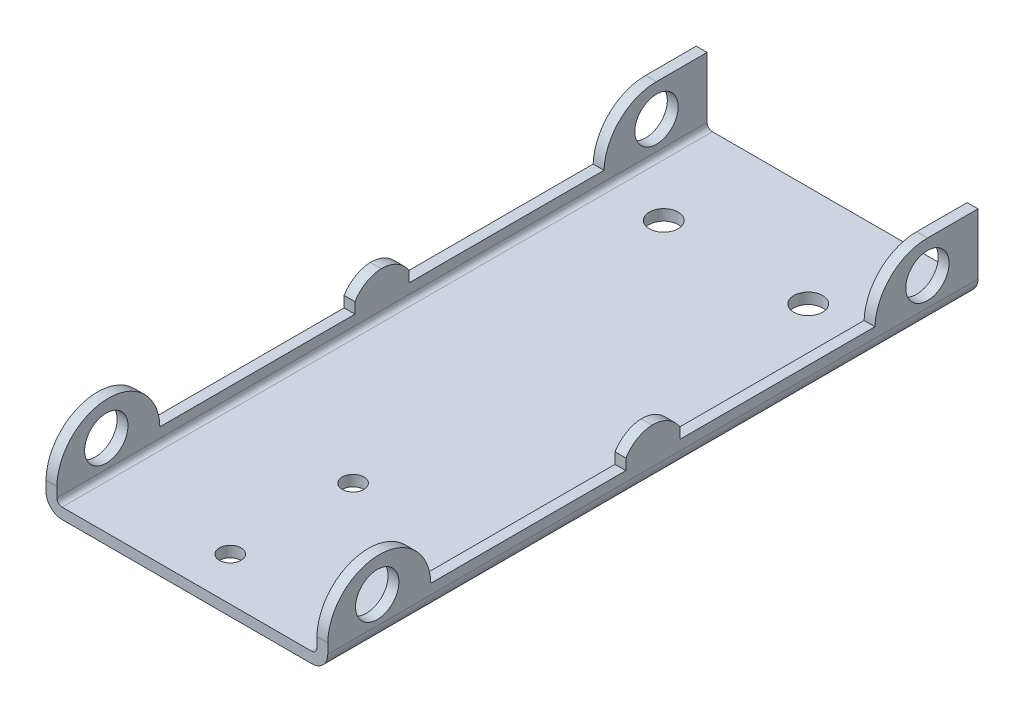
SolidWorks part; units mm, degrees
ref_plane "Front Plane" through (0, 0, 0) normal (0, 0, 1) x (1, 0, 0)
ref_plane "Top Plane" through (0, 0, 0) normal (0, 1, 0) x (1, 0, 0)
ref_plane "Right Plane" through (0, 0, 0) normal (1, 0, 0) x (0, 0, -1)
other "Configuration Table"
ref_plane "Plane1" through (-29, 0, 0) normal (-1, 0, 0) x (0, -1, 0)
sketch "Sketch1" plane through (-29, 0, 0) normal (-1, 0, 0) x (0, -1, 0)
  line L0 (-9.1381, -90) -> (1.5, -90)
  line L1 (1.5, -90) -> (1.5, 0)
  line L2 (1.5, 0) -> (-2.1289, 0)
  line L3 (-2.1289, -14.2617) -> (-2.1289, -41.2617)
  line L4 (-2.1289, -41.2617) -> (-3.6289, -41.2617)
  line L5 (-3.6383, -48.7314) -> (-2.1381, -48.7314)
  line L6 (-2.1381, -48.7314) -> (-2.1381, -75.7314)
  line L7 (-9.1381, -83) -> (-9.1381, -90)
  arc A0 (-2.1289, 0) -> (-2.1289, -14.2617) centre (-1.998, -7.1309) ccw
  arc A1 (-3.6289, -41.2617) -> (-5.7783, -44.8732) centre (-1.2572, -45.1185) ccw
  arc A2 (-5.7783, -44.8732) -> (-3.6383, -48.7314) centre (-1.2506, -44.8845) ccw
  arc A3 (-2.1381, -75.7314) -> (-9.1381, -83) centre (-1.8643, -83) ccw
extrude "Boss-Extrude1" add sketch "Sketch1" against normal blind 1.5
sketch "Sketch2" plane through (-27.5, 0, 0) normal (1, 0, 0) x (0, 0, -1)
  line L0 (0, 0) -> (90, 0)
  line L1 (90, 0) -> (90, -1.5)
  line L2 (90, -1.5) -> (0, -1.5)
  line L3 (0, -1.5) -> (0, 0)
extrude "Boss-Extrude2" add sketch "Sketch2" along normal blind 36
sketch "Sketch3" plane through (8.5, 0, 0) normal (1, 0, 0) x (0, 0, -1)
  line L0 (0, -1.5) -> (0, 2.1289)
  line L1 (14.2617, 2.1289) -> (41.2617, 2.1289)
  line L2 (41.2617, 2.1289) -> (41.2617, 3.6289)
  line L3 (48.7314, 3.6383) -> (48.7314, 2.1381)
  line L4 (48.7314, 2.1381) -> (75.7314, 2.1381)
  line L5 (83, 9.1381) -> (90, 9.1381)
  line L6 (90, 9.1381) -> (90, -1.5)
  line L7 (90, -1.5) -> (0, -1.5)
  arc A0 (0, 2.1289) -> (14.2617, 2.1289) centre (7.1309, 1.998) cw
  arc A1 (41.2617, 3.6289) -> (44.8732, 5.7783) centre (45.1185, 1.2572) cw
  arc A2 (44.8732, 5.7783) -> (48.7314, 3.6383) centre (44.8845, 1.2506) cw
  arc A3 (75.7314, 2.1381) -> (83, 9.1381) centre (83, 1.8643) cw
extrude "Boss-Extrude3" add sketch "Sketch3" along normal blind 1.5
hole_wizard "Ø6.0 (6) Diameter Hole1" positions "Sketch5" profile "Sketch4" hole size "Ø6.0" standard "ANSI Metric"
sketch "Sketch5" plane through (8.5, 0, 0) normal (-1, 0, 0) x (0, 0, 1)
  point P0 (-6.8458, 4.4817)
  point P1 (-83, 4.6381)
sketch "Sketch4" plane through (8.5, 4.4817, -6.8458) normal (0, 1, 0) x (0, 0, 1)
  line L0 (0, 0) -> (0, 1.5)
  line L1 (0, 1.5) -> (3, 1.5)
  line L2 (3, 1.5) -> (3, 0)
  line L5 (3, 0) -> (0, 0)
  line L11 (0, -6.35) -> (0, 107.95) construction
  dimension "通孔孔直径" = 6
  dimension "通孔孔深度" = 1.5
hole_wizard "Ø6.0 (6) Diameter Hole2" positions "Sketch7" profile "Sketch6" hole size "Ø6.0" standard "ANSI Metric"
sketch "Sketch7" plane through (-27.5, 0, 0) normal (1, 0, 0) x (0, 0, -1)
  point P0 (83, 4.6381)
  point P1 (6.8458, 4.4817)
sketch "Sketch6" plane through (-27.5, 4.6381, -83) normal (0, 1, 0) x (0, 0, -1)
  line L0 (0, 0) -> (0, 1.5)
  line L1 (0, 1.5) -> (3, 1.5)
  line L2 (3, 1.5) -> (3, 0)
  line L5 (3, 0) -> (0, 0)
  line L11 (0, -6.35) -> (0, 107.95) construction
  dimension "通孔孔直径" = 6
  dimension "通孔孔深度" = 1.5
hole_wizard "Ø4.0 (4) Diameter Hole1" positions "Sketch9" profile "Sketch8" hole size "Ø4.0" standard "ANSI Metric"
sketch "Sketch9" plane through (0, 0, 0) normal (0, 1, 0) x (1, 0, 0)
  point P0 (-19.5, 76)
  point P1 (0.5, 76)
sketch "Sketch8" plane through (-19.5, 0, -76) normal (1, 0, 0) x (0, 0, 1)
  line L0 (0, 0) -> (0, 1.5)
  line L1 (0, 1.5) -> (2, 1.5)
  line L2 (2, 1.5) -> (2, 0)
  line L5 (2, 0) -> (0, 0)
  line L11 (0, -6.35) -> (0, 107.95) construction
  dimension "通孔孔直径" = 4
  dimension "通孔孔深度" = 1.5
hole_wizard "Ø3.0 (3) Diameter Hole1" positions "Sketch11" profile "Sketch10" hole size "Ø3.0" standard "ANSI Metric"
sketch "Sketch11" plane through (0, 0, 0) normal (0, 1, 0) x (1, 0, 0)
  point P0 (-9.5, 6)
  point P1 (-9.5, 23)
sketch "Sketch10" plane through (-9.5, 0, -6) normal (1, 0, 0) x (0, 0, 1)
  line L0 (0, 0) -> (0, 1.5)
  line L1 (0, 1.5) -> (1.5, 1.5)
  line L2 (1.5, 1.5) -> (1.5, 0)
  line L5 (1.5, 0) -> (0, 0)
  line L11 (0, -6.35) -> (0, 107.95) construction
  dimension "通孔孔直径" = 3
  dimension "通孔孔深度" = 1.5
fillet "Fillet1" radius 0.7366 2 edges at (-27.5, 0, -45) (8.5, 0, -45)
fillet "Fillet2" radius 2.2366 2 edges at (-29, -1.5, -45) (10, -1.5, -45)
